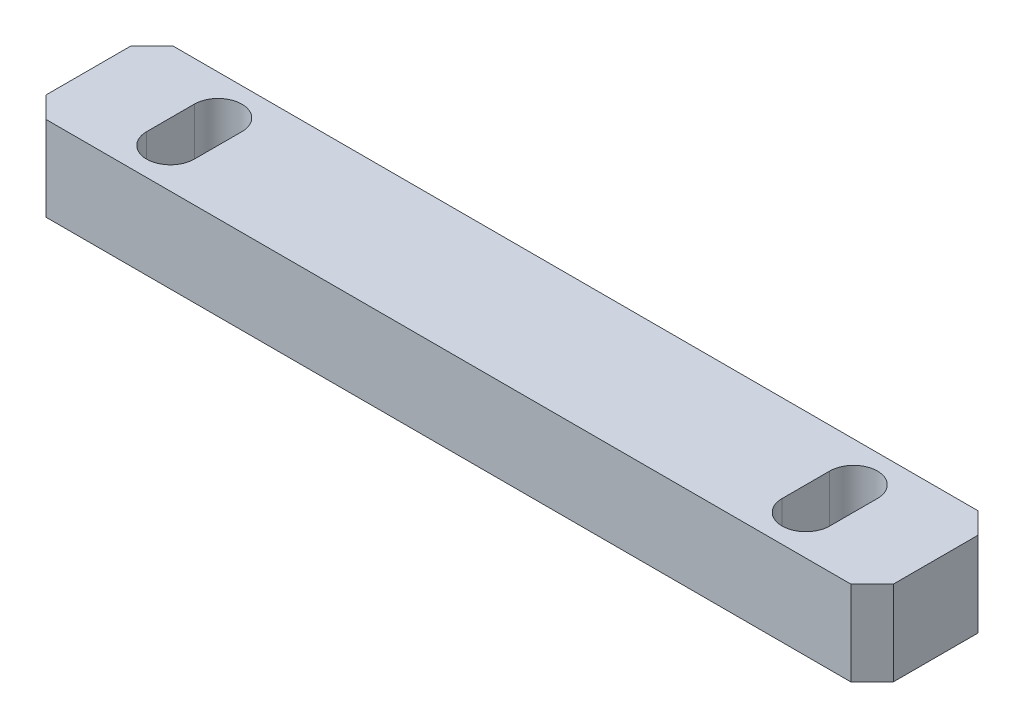
from build123d import *

# Parameters (mm, degrees)
SKETCH1_W           = 80
SKETCH1_H           = 12
BOSS_EXTRUDE1_DEPTH = 8
CHAMFER1_SIZE       = 2
SKETCH2_R           = 2.25
CUT_EXTRUDE1_DEPTH  = 10
CUT_EXTRUDE2_DEPTH  = 10


with BuildPart() as part:
    # Sketch1 → Boss-Extrude1 (new body)
    with BuildSketch(Plane(origin=(0, 0, 0), x_dir=(1, 0, 0), z_dir=(0, 1, 0))):
        with Locations((40, 6)):
            Rectangle(SKETCH1_W, SKETCH1_H)
    extrude(amount=BOSS_EXTRUDE1_DEPTH)

    # Chamfer1
    chamfer1_edges = [part.edges().sort_by_distance(p)[0] for p in [
        (0, 4, -12),
        (80, 4, -12),
        (80, 4, 0),
        (0, 4, 0),
    ]]
    chamfer(chamfer1_edges, length=CHAMFER1_SIZE)

    # Sketch2 → Cut-Extrude1 (cut)
    with BuildSketch(Plane.XZ):
        with Locations(Location((10, -6, 0), (0, 0, 270))):
            Circle(SKETCH2_R)
        with Locations(Location((70, -6, 0), (0, 0, 270))):
            Circle(SKETCH2_R)
    extrude(amount=-CUT_EXTRUDE1_DEPTH, mode=Mode.SUBTRACT)

    # Sketch4 → Cut-Extrude2 (cut)
    with BuildSketch(Plane.XZ):
        with BuildLine():
            Line((7.75, -8.25), (7.75, -3.75))
            ThreePointArc((7.75, -3.75), (10, -1.5), (12.25, -3.75))
            Line((12.25, -3.75), (12.25, -8.25))
            ThreePointArc((12.25, -8.25), (10, -10.5), (7.75, -8.25))
        make_face()
        with BuildLine():
            Line((72.25, -8.25), (72.25, -3.75))
            ThreePointArc((72.25, -3.75), (70, -1.5), (67.75, -3.75))
            Line((67.75, -3.75), (67.75, -8.25))
            ThreePointArc((67.75, -8.25), (70, -10.5), (72.25, -8.25))
        make_face()
    extrude(amount=-CUT_EXTRUDE2_DEPTH, mode=Mode.SUBTRACT)


solid = part.part
